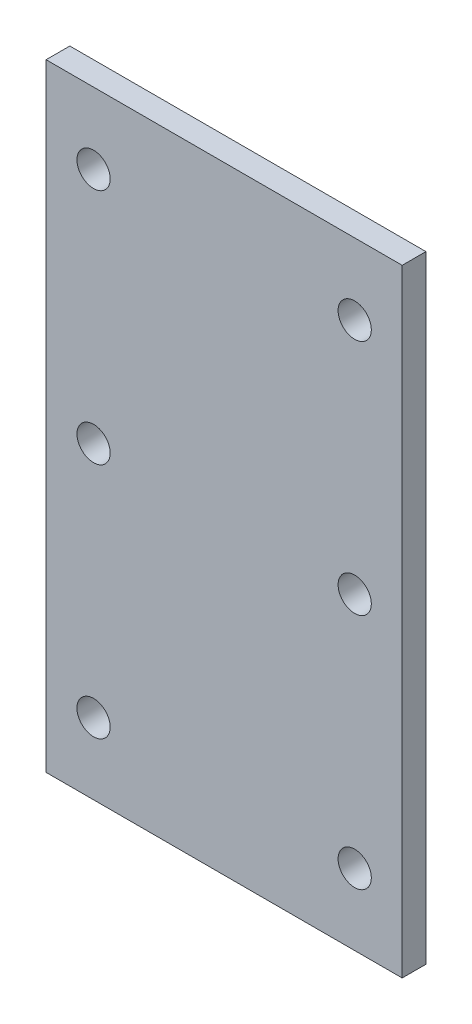
from build123d import *

# Parameters (mm, degrees)
SKETCH1_W                  = 150
SKETCH1_H                  = 260
BOSS_EXTRUDE1_DEPTH        = 10
F_14_0_14_DIAMETER_HOLE1_D = 14


with BuildPart() as part:
    # Sketch1 → Boss-Extrude1 (new body)
    with BuildSketch(Plane.XY):
        Rectangle(SKETCH1_W, SKETCH1_H)
    extrude(amount=BOSS_EXTRUDE1_DEPTH)

    # Ø14.0 (14) Diameter Hole1 (through all)
    with Locations(Plane.XY.offset(10)):
        with Locations((-55, 100), (-55, 0), (-55, -100), (55, -100), (55, 0), (55, 100)):
            Hole(F_14_0_14_DIAMETER_HOLE1_D / 2)


solid = part.part
